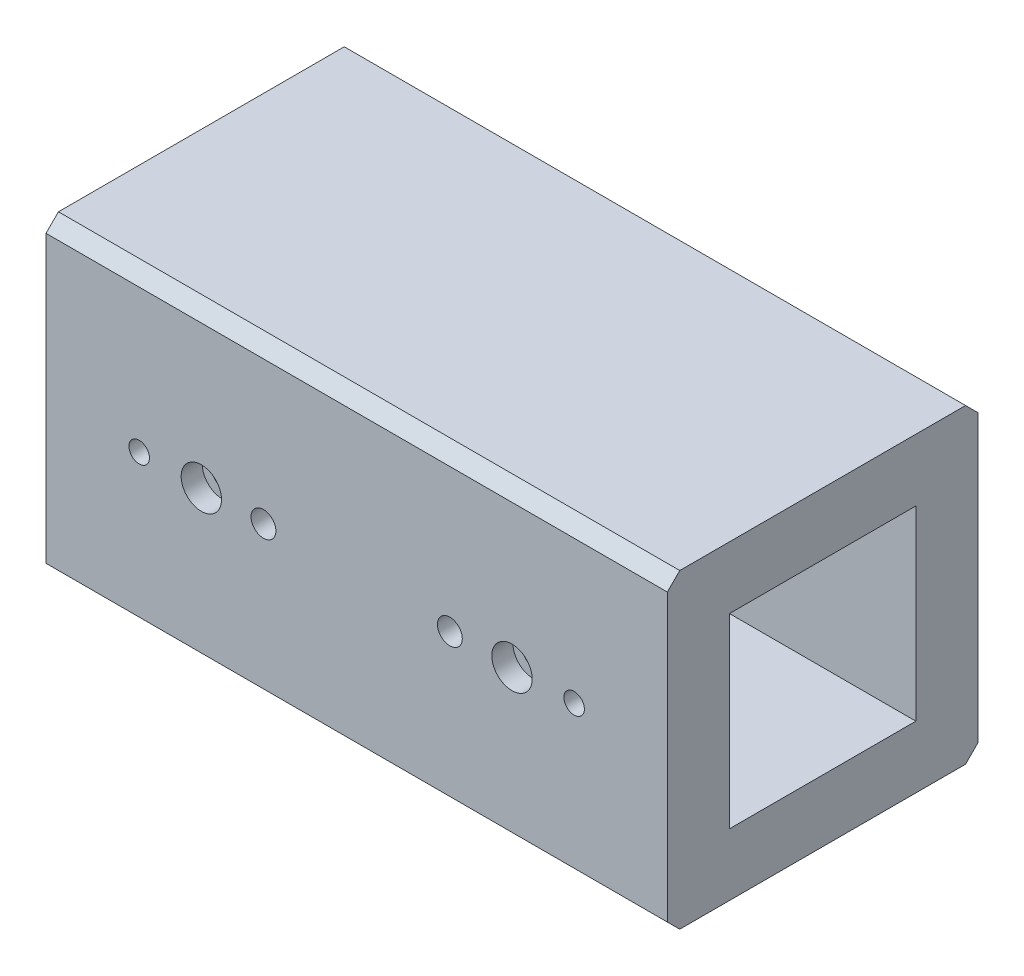
from build123d import *

# Parameters (mm, degrees)
SKETCH1_W                                           = 100
SKETCH1_H                                           = 50
BOSS_EXTRUDE1_DEPTH                                 = 50
SKETCH2_W                                           = 30
SKETCH2_H                                           = 30
CUT_EXTRUDE1_DEPTH                                  = 115.564392374
CBORE_FOR_M3_HEX_SOCKET_HEAD_CAP_SCREW1_D           = 2
CBORE_FOR_M3_HEX_SOCKET_HEAD_CAP_SCREW1_DEPTH       = 10
CBORE_FOR_M3_HEX_SOCKET_HEAD_CAP_SCREW1_CBORE_D     = 6.5
CBORE_FOR_M3_HEX_SOCKET_HEAD_CAP_SCREW1_CBORE_DEPTH = 3.4
CBORE_FOR_M3_HEX_SOCKET_HEAD_CAP_SCREW2_D           = 2
CBORE_FOR_M3_HEX_SOCKET_HEAD_CAP_SCREW2_CBORE_D     = 6.5
CBORE_FOR_M3_HEX_SOCKET_HEAD_CAP_SCREW2_CBORE_DEPTH = 3.4
M4_TAPPED_HOLE1_D                                   = 3.3
M4_TAPPED_HOLE1_DEPTH                               = 10.1
M4_TAPPED_HOLE1_TIP                                 = 0.991420021
F_4_0_4_DIAMETER_HOLE1_D                            = 4
F_4_0_4_DIAMETER_HOLE1_DEPTH                        = 10
CHAMFER1_SIZE                                       = 2
M8_TAPPED_HOLE1_D                                   = 6.8
M8_TAPPED_HOLE1_DEPTH                               = 19.75
M8_TAPPED_HOLE1_TIP                                 = 2.042926105
M4_TAPPED_HOLE2_D                                   = 3.3
M4_TAPPED_HOLE2_DEPTH                               = 10.1
M4_TAPPED_HOLE2_TIP                                 = 0.991420021
M4_TAPPED_HOLE3_D                                   = 3.3
M4_TAPPED_HOLE3_DEPTH                               = 10.1
M4_TAPPED_HOLE3_TIP                                 = 0.991420021


with BuildPart() as part:
    # Sketch1 → Boss-Extrude1 (new body)
    with BuildSketch(Plane.XY):
        Rectangle(SKETCH1_W, SKETCH1_H)
    extrude(amount=BOSS_EXTRUDE1_DEPTH)

    # Sketch2 → Cut-Extrude1 (cut, through all)
    with BuildSketch(Plane(origin=(50, 0, 0), x_dir=(0, 0, -1), z_dir=(1, 0, 0))):
        with Locations((-25, 0)):
            Rectangle(SKETCH2_W, SKETCH2_H)
    extrude(amount=-CUT_EXTRUDE1_DEPTH, mode=Mode.SUBTRACT)

    # CBORE for M3 Hex Socket Head Cap Screw1
    with Locations(Plane(origin=(0, 0, 0), x_dir=(-1, 0, 0), z_dir=(0, 0, -1))):
        with Locations((-25, 0), (25, 0)):
            CounterBoreHole(CBORE_FOR_M3_HEX_SOCKET_HEAD_CAP_SCREW1_D / 2, CBORE_FOR_M3_HEX_SOCKET_HEAD_CAP_SCREW1_CBORE_D / 2, CBORE_FOR_M3_HEX_SOCKET_HEAD_CAP_SCREW1_CBORE_DEPTH, depth=CBORE_FOR_M3_HEX_SOCKET_HEAD_CAP_SCREW1_DEPTH)

    # CBORE for M3 Hex Socket Head Cap Screw2 (through all)
    with Locations(Plane.XY.offset(50)):
        with Locations((-25, 0), (25, 0)):
            CounterBoreHole(CBORE_FOR_M3_HEX_SOCKET_HEAD_CAP_SCREW2_D / 2, CBORE_FOR_M3_HEX_SOCKET_HEAD_CAP_SCREW2_CBORE_D / 2, CBORE_FOR_M3_HEX_SOCKET_HEAD_CAP_SCREW2_CBORE_DEPTH)

    # M4 Tapped Hole1
    with Locations(Plane.XY.offset(50)):
        with Locations((-35, 0), (35, 0)):
            Hole(M4_TAPPED_HOLE1_D / 2, depth=M4_TAPPED_HOLE1_DEPTH)
            with Locations((0, 0, -(M4_TAPPED_HOLE1_DEPTH + M4_TAPPED_HOLE1_TIP / 2))):  # 118° drill point
                Cone(0, M4_TAPPED_HOLE1_D / 2, M4_TAPPED_HOLE1_TIP, mode=Mode.SUBTRACT)

    # Ø4.0 (4) Diameter Hole1
    with Locations(Plane.XY.offset(50)):
        with Locations((15, 0), (-15, 0)):
            Hole(F_4_0_4_DIAMETER_HOLE1_D / 2, depth=F_4_0_4_DIAMETER_HOLE1_DEPTH)

    # Chamfer1
    chamfer1_edges = [part.edges().sort_by_distance(p)[0] for p in [
        (0, -25, 50),
        (0, -25, 0),
        (0, 25, 0),
        (0, 25, 50),
    ]]
    chamfer(chamfer1_edges, length=CHAMFER1_SIZE)

    # M8 Tapped Hole1
    with Locations(Plane(origin=(0, -25, 0), x_dir=(-1, 0, 0), z_dir=(0, -1, 0))):
        with Locations((0, -25)):
            Hole(M8_TAPPED_HOLE1_D / 2, depth=M8_TAPPED_HOLE1_DEPTH)
            with Locations((0, 0, -(M8_TAPPED_HOLE1_DEPTH + M8_TAPPED_HOLE1_TIP / 2))):  # 118° drill point
                Cone(0, M8_TAPPED_HOLE1_D / 2, M8_TAPPED_HOLE1_TIP, mode=Mode.SUBTRACT)

    # M4 Tapped Hole2
    with Locations(Plane(origin=(0, 0, 3.4), x_dir=(-1, 0, 0), z_dir=(0, 0, -1))):
        with Locations((-25, 0), (25, 0)):
            Hole(M4_TAPPED_HOLE2_D / 2, depth=M4_TAPPED_HOLE2_DEPTH)
            with Locations((0, 0, -(M4_TAPPED_HOLE2_DEPTH + M4_TAPPED_HOLE2_TIP / 2))):  # 118° drill point
                Cone(0, M4_TAPPED_HOLE2_D / 2, M4_TAPPED_HOLE2_TIP, mode=Mode.SUBTRACT)

    # M4 Tapped Hole3
    with Locations(Plane.XY.offset(46.6)):
        with Locations((-25, 0), (25, 0)):
            Hole(M4_TAPPED_HOLE3_D / 2, depth=M4_TAPPED_HOLE3_DEPTH)
            with Locations((0, 0, -(M4_TAPPED_HOLE3_DEPTH + M4_TAPPED_HOLE3_TIP / 2))):  # 118° drill point
                Cone(0, M4_TAPPED_HOLE3_D / 2, M4_TAPPED_HOLE3_TIP, mode=Mode.SUBTRACT)


solid = part.part
